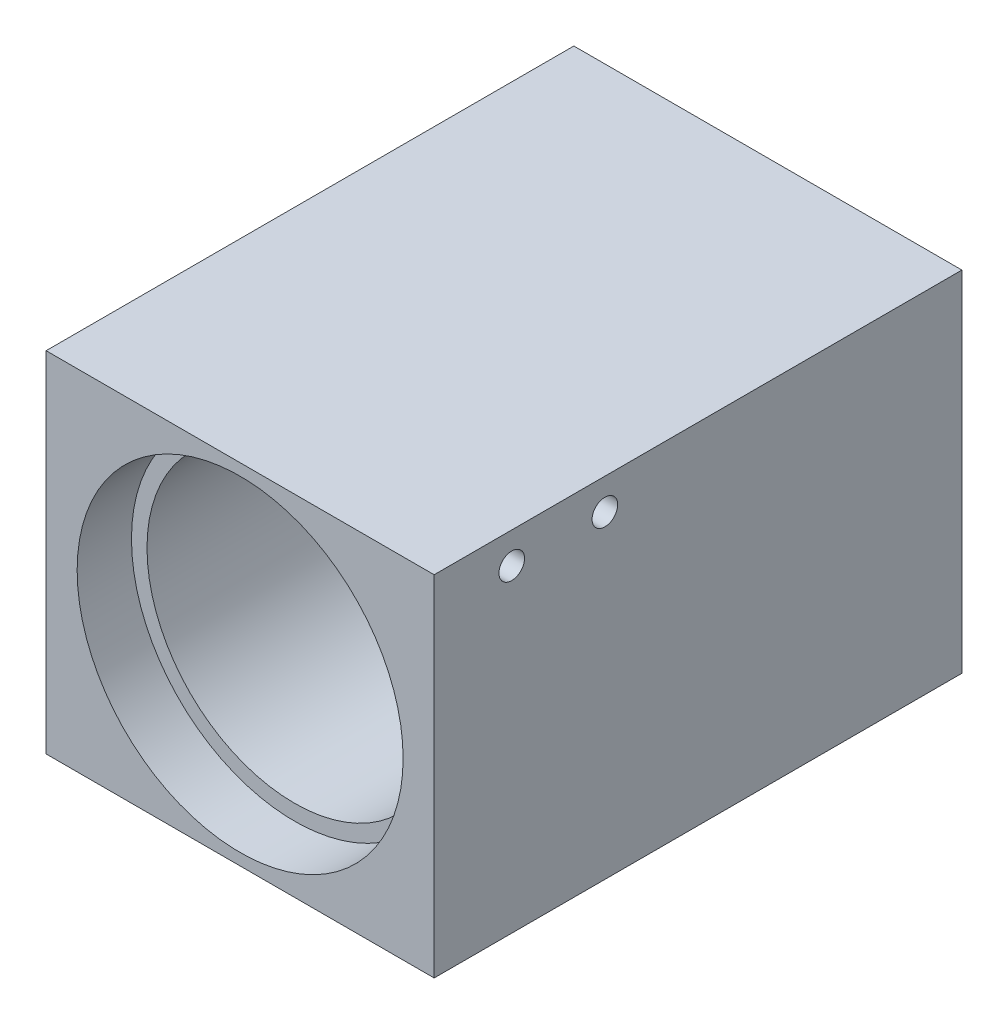
from build123d import *

# Parameters (mm, degrees)
SKETCH_1_W                  = 50
SKETCH_1_H                  = 45
EXTRUDE_1_DEPTH             = 68
SKETCH_2_R                  = 19
CUT_EXTRUDE_1_DEPTH         = 79
SKETCH_3_R                  = 21
CUT_EXTRUDE_2_DEPTH         = 7
CUT_EXTRUDE_START           = -25
SKETCH_4_R                  = 21
CUT_EXTRUDE_3_DEPTH         = 25
HOLE_WIZARD_M4_1_D          = 3.3
HOLE_WIZARD_M4_1_DEPTH      = 10.1
HOLE_WIZARD_M4_1_TIP        = 0.991420021
HOLE_WIZARD_M4_2_D          = 3.3
HOLE_WIZARD_M4_2_DEPTH      = 10.1
HOLE_WIZARD_M4_2_TIP        = 0.991420021
HOLE_WIZARD_6_5_6_5_1_D     = 6.5
HOLE_WIZARD_6_5_6_5_1_DEPTH = 20
HOLE_WIZARD_6_5_6_5_1_TIP   = 1.952797012
HOLE_WIZARD_M4_4_D          = 3.3
HOLE_WIZARD_M4_4_DEPTH      = 10.1
HOLE_WIZARD_M4_4_TIP        = 0.991420021


with BuildPart() as part:
    # 草图1 → 凸台-拉伸1 (new body)
    with BuildSketch(Plane.XY):
        with Locations((25, 22.5)):
            Rectangle(SKETCH_1_W, SKETCH_1_H)
    extrude(amount=EXTRUDE_1_DEPTH)

    # 草图2 → 切除-拉伸1 (cut)
    with BuildSketch(Plane(origin=(0, 0, 0), x_dir=(-1, 0, 0), z_dir=(0, 0, -1))):
        with Locations((-25, 22.5)):
            Circle(SKETCH_2_R)
    extrude(amount=-CUT_EXTRUDE_1_DEPTH, mode=Mode.SUBTRACT)

    # 草图3 → 切除-拉伸2 (cut)
    with BuildSketch(Plane.XY.offset(68)):
        with Locations((25, 22.5)):
            Circle(SKETCH_3_R)
    extrude(amount=-CUT_EXTRUDE_2_DEPTH, mode=Mode.SUBTRACT)

    # 草图4 → 切除-拉伸3 (cut)
    with BuildSketch(Plane(origin=(0, 0, 0), x_dir=(-1, 0, 0), z_dir=(0, 0, -1)).offset(CUT_EXTRUDE_START)):
        with Locations(Location((-25, 22.5, 0), (0, 0, 180))):
            Circle(SKETCH_4_R)
    extrude(amount=CUT_EXTRUDE_3_DEPTH, mode=Mode.SUBTRACT)

    # M4 螺纹孔1
    with Locations(Plane(origin=(50, 0, 0), x_dir=(0, 0, -1), z_dir=(1, 0, 0))):
        with Locations((-58, 41), (-46, 41)):
            Hole(HOLE_WIZARD_M4_1_D / 2, depth=HOLE_WIZARD_M4_1_DEPTH)
            with Locations((0, 0, -(HOLE_WIZARD_M4_1_DEPTH + HOLE_WIZARD_M4_1_TIP / 2))):  # 118° drill point
                Cone(0, HOLE_WIZARD_M4_1_D / 2, HOLE_WIZARD_M4_1_TIP, mode=Mode.SUBTRACT)

    # M4 螺纹孔2
    with Locations(Plane.ZY):
        with Locations((46, 41), (58, 41)):
            Hole(HOLE_WIZARD_M4_2_D / 2, depth=HOLE_WIZARD_M4_2_DEPTH)
            with Locations((0, 0, -(HOLE_WIZARD_M4_2_DEPTH + HOLE_WIZARD_M4_2_TIP / 2))):  # 118° drill point
                Cone(0, HOLE_WIZARD_M4_2_D / 2, HOLE_WIZARD_M4_2_TIP, mode=Mode.SUBTRACT)

    # Ø6.5 (6.5) 直径孔1
    with Locations(Plane(origin=(0, 0, 0), x_dir=(-1, 0, 0), z_dir=(0, -1, 0))):
        with Locations((-25, -38)):
            Hole(HOLE_WIZARD_6_5_6_5_1_D / 2, depth=HOLE_WIZARD_6_5_6_5_1_DEPTH)
            with Locations((0, 0, -(HOLE_WIZARD_6_5_6_5_1_DEPTH + HOLE_WIZARD_6_5_6_5_1_TIP / 2))):  # 118° drill point
                Cone(0, HOLE_WIZARD_6_5_6_5_1_D / 2, HOLE_WIZARD_6_5_6_5_1_TIP, mode=Mode.SUBTRACT)

    # M4 螺纹孔4
    with Locations(Plane(origin=(0, 0, 0), x_dir=(-1, 0, 0), z_dir=(0, 0, -1))):
        with Locations((-5, 36.5), (-45, 36.5), (-45, 8.5), (-5, 8.5)):
            Hole(HOLE_WIZARD_M4_4_D / 2, depth=HOLE_WIZARD_M4_4_DEPTH)
            with Locations((0, 0, -(HOLE_WIZARD_M4_4_DEPTH + HOLE_WIZARD_M4_4_TIP / 2))):  # 118° drill point
                Cone(0, HOLE_WIZARD_M4_4_D / 2, HOLE_WIZARD_M4_4_TIP, mode=Mode.SUBTRACT)


solid = part.part
